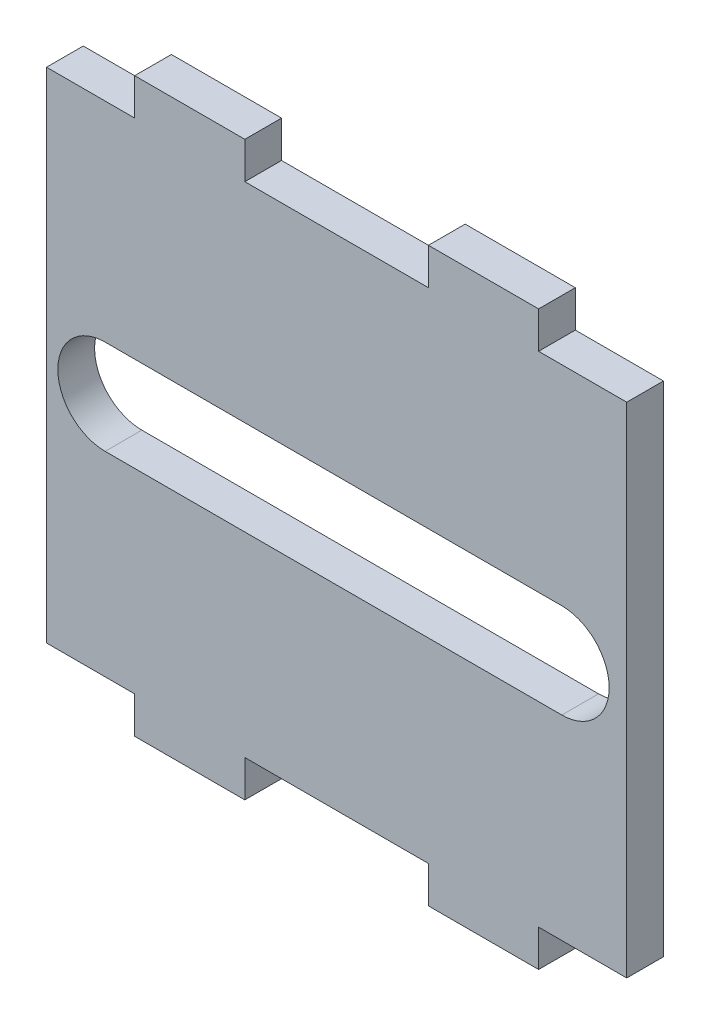
from build123d import *

# Parameters (mm, degrees)
EXTRUDE_1_DEPTH     = 5
CUT_EXTRUDE_2_DEPTH = 5


with BuildPart() as part:
    # 草图1 → 凸台-拉伸1 (new body)
    with BuildSketch(Plane.XY):
        Polygon((12, 0), (27, 0), (27, 5), (52, 5), (52, 0), (67, 0), (67, 5), (79, 5), (79, 72.9), (67, 72.9), (67, 77.9), (52, 77.9), (52, 72.9), (27, 72.9), (27, 77.9), (12, 77.9), (12, 72.9), (0, 72.9), (0, 5), (12, 5), align=None)
    extrude(amount=EXTRUDE_1_DEPTH)

    # 草图2 → 切除-拉伸2 (cut)
    with BuildSketch(Plane(origin=(0, 0, 0), x_dir=(-1, 0, 0), z_dir=(0, 0, -1))):
        with BuildLine():
            Line((-70.163147459, 44.470964867), (-7.979563682, 44.470964867))
            ThreePointArc((-7.979563682, 44.470964867), (-1.539904649, 38.031305835), (-7.979563682, 31.591646802))
            Line((-7.979563682, 31.591646802), (-70.163147459, 31.591646802))
            ThreePointArc((-70.163147459, 31.591646802), (-76.602806492, 38.031305835), (-70.163147459, 44.470964867))
        make_face()
    extrude(amount=-CUT_EXTRUDE_2_DEPTH, mode=Mode.SUBTRACT)


solid = part.part
